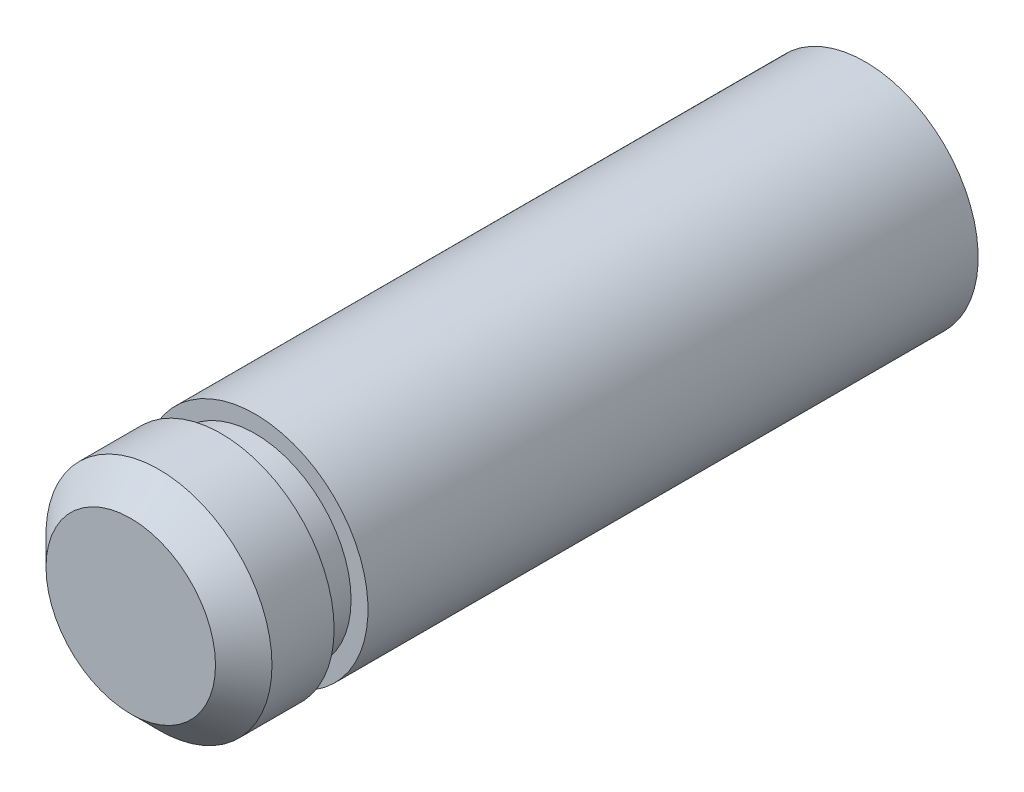
SolidWorks part; units mm, degrees
ref_plane "Front Plane" through (0, 0, 0) normal (0, 0, 1) x (1, 0, 0)
ref_plane "Top Plane" through (0, 0, 0) normal (0, 1, 0) x (1, 0, 0)
ref_plane "Right Plane" through (0, 0, 0) normal (1, 0, 0) x (0, 0, -1)
other "Configuration Table"
sketch "Sketch1" plane through (0, 0, 0) normal (0, 0, 1) x (1, 0, 0)
  circle A0 centre (0, 0) radius 2
  dimension "D1" = 4
extrude "Boss-Extrude1" add sketch "Sketch1" along normal blind 10.8
sketch "Sketch2" plane through (0, 0, 10.8) normal (0, 0, 1) x (1, 0, 0)
  circle A0 centre (0, 0) radius 1.7
  dimension "D1" = 3.4
extrude "Boss-Extrude2" add sketch "Sketch2" along normal blind 0.6
sketch "Sketch3" plane through (0, 0, 11.4) normal (0, 0, 1) x (1, 0, 0)
  circle A0 centre (0, 0) radius 2 construction
  circle A1 centre (0, 0) radius 2
extrude "Boss-Extrude3" add sketch "Sketch3" along normal blind 1.6
chamfer "Chamfer1" distance 0.5 angle 45 1 edges at (2, 0, 13)
